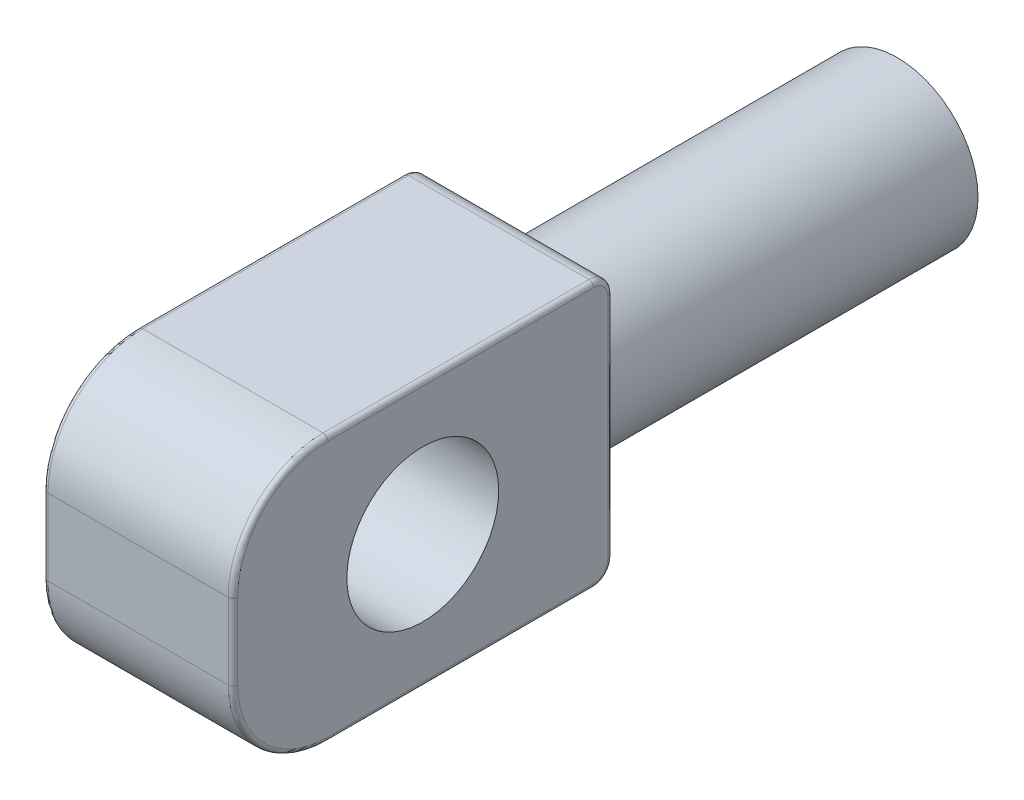
SolidWorks part; units mm, degrees
ref_plane "Front Plane" through (0, 0, 0) normal (0, 0, 1) x (1, 0, 0)
ref_plane "Top Plane" through (0, 0, 0) normal (0, 1, 0) x (1, 0, 0)
ref_plane "Right Plane" through (0, 0, 0) normal (1, 0, 0) x (0, 0, -1)
sketch "Sketch1" plane through (0, 0, 0) normal (0, 0, 1) x (1, 0, 0)
  circle A0 centre (0, 0) radius 4.25
  dimension "D1" = 8.5
extrude "Boss-Extrude1" add sketch "Sketch1" along normal blind 20
sketch "Sketch2" plane through (0, 0, 0) normal (1, 0, 0) x (0, 0, -1)
  line L0 (0, 0) -> (-40.0049, 0) construction
  line L1 (-21.0049, -7) -> (-35.0049, -7)
  line L2 (-20.0049, -6) -> (-20.0049, 6)
  line L3 (-21.0049, 7) -> (-35.0049, 7)
  line L4 (-40.0049, -2) -> (-40.0049, 2)
  arc A0 (-35.0049, -7) -> (-40.0049, -2) centre (-35.0049, -2) cw
  arc A1 (-35.0049, 7) -> (-40.0049, 2) centre (-35.0049, 2) ccw
  arc A2 (-21.0049, -7) -> (-20.0049, -6) centre (-21.0049, -6) ccw
  arc A3 (-20.0049, 6) -> (-21.0049, 7) centre (-21.0049, 6) ccw
  point P11 (-40.0049, 7)
  point P14 (-20.0049, -7)
  point P17 (-20.0049, 7)
  dimension "D4" = 5
  dimension "D5" = 1
  dimension "D1" = 14
  dimension "D2" = 20
  dimension "D3" = 20.0049
extrude "Boss-Extrude2" add sketch "Sketch2" along normal mid plane 10 separate body
fillet "Fillet1" radius 0.25 16 edges at (-5, -7, 28.0049) (-5, -6.7071, 20.2978) (-5, 0, 20.0049) (-5, 6.7071, 20.2978) (-5, 7, 28.0049) (-5, 5.5355, 38.5404) (-5, 0, 40.0049) (-5, -5.5355, 38.5404) (5, 0, 40.0049) (5, 5.5355, 38.5404) (5, 7, 28.0049) (5, 6.7071, 20.2978) (5, 0, 20.0049) (5, -6.7071, 20.2978) (5, -7, 28.0049) (5, -5.5355, 38.5404)
hole_wizard "M3.5 Tapped Hole1" positions "Sketch3" profile "Sketch4" tap size "M3.5" standard "ISO"
sketch "Sketch3" plane through (0, 0, 0) normal (0, 0, -1) x (-1, 0, 0)
  point P0 (0, 0)
sketch "Sketch4" plane through (0, 0, 0) normal (1, 0, 0) x (0, 1, 0)
  line L0 (0, 0) -> (0, 10.8712)
  line L1 (0, 10.8712) -> (1.45, 10)
  line L2 (1.45, 10) -> (1.45, 0.325)
  line L3 (1.45, 0.325) -> (1.775, 0)
  line L5 (1.775, 0) -> (0, 0)
  line L6 (-1.45, 0.325) -> (-1.775, 0) construction
  line L10 (0, 10.8712) -> (-1.45, 10) construction
  line L11 (0, -6.35) -> (0, 107.95) construction
  dimension "Tap Drill Dia." = 2.9
  dimension "Tap Drill Depth" = 10
  dimension "Near C'Sink Dia." = 3.55
  dimension "Near C'Sink Angle" = 90
  dimension "Drill Angle" = 118
cosmetic thread "Hole Thread1" parameters "D1"=7, "D2"=3.5
sketch "Sketch5" plane through (5, 0, 0) normal (1, 0, 0) x (0, 0, -1)
  line L0 (-40.0049, 0) -> (-20.0049, 0) construction
  line L1 (-40.0049, -2) -> (-40.0049, 2) construction
  line L2 (-20.0049, 6) -> (-20.0049, -6) construction
  circle A0 centre (-30.0049, 0) radius 4
  dimension "D1" = 8
extrude "Cut-Extrude1" cut sketch "Sketch5" against normal up to next (10 mm away)
